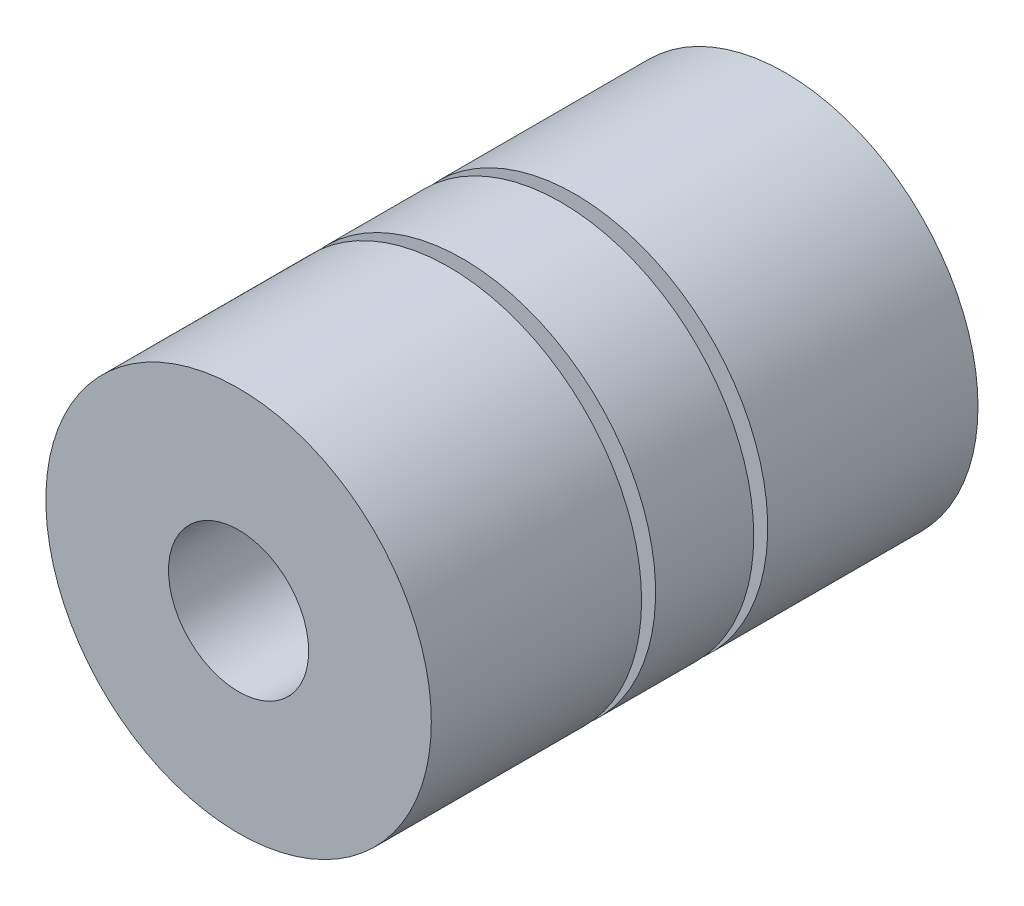
SolidWorks part; units mm, degrees
ref_plane "Front Plane" through (0, 0, 0) normal (0, 0, 1) x (1, 0, 0)
ref_plane "Top Plane" through (0, 0, 0) normal (0, 1, 0) x (1, 0, 0)
ref_plane "Right Plane" through (0, 0, 0) normal (1, 0, 0) x (0, 0, -1)
sketch "Sketch1" plane through (0, 0, 0) normal (0, 0, 1) x (1, 0, 0)
  circle A0 centre (0, 0) radius 27.5
  dimension "D1" = 55
extrude "Boss-Extrude1" add sketch "Sketch1" along normal blind 78
sketch "Sketch2" plane through (0, 0, 78) normal (0, 0, 1) x (1, 0, 0)
  circle A0 centre (0, 0) radius 10
  dimension "D1" = 20
extrude "Cut-Extrude1" cut sketch "Sketch2" against normal blind 30
sketch "Sketch3" plane through (0, 0, 0) normal (0, 0, -1) x (-1, 0, 0)
  circle A0 centre (0, 0) radius 9.5
  dimension "D1" = 19
extrude "Cut-Extrude2" cut sketch "Sketch3" against normal blind 30
sketch "Sketch4" plane through (0, 0, 0) normal (0, 1, 0) x (1, 0, 0)
  line L0 (-27.5, -39) -> (49.7456, -39) construction
  line L1 (-29.7585, -30) -> (31.5351, -30)
  line L2 (-29.7585, -30) -> (-29.7585, -32)
  line L3 (-29.7585, -32) -> (31.5351, -32)
  line L4 (31.5351, -30) -> (31.5351, -32)
  line L5 (-27.5, 0) -> (-27.5, -78) construction
  line L6 (31.5351, -48) -> (31.5351, -46)
  line L7 (-29.7585, -46) -> (31.5351, -46)
  line L8 (-29.7585, -48) -> (-29.7585, -46)
  line L9 (-29.7585, -48) -> (31.5351, -48)
  dimension "D1" = 2
  dimension "D2" = 7
extrude "Cut-Extrude3" cut sketch "Sketch4" against normal mid plane 60
